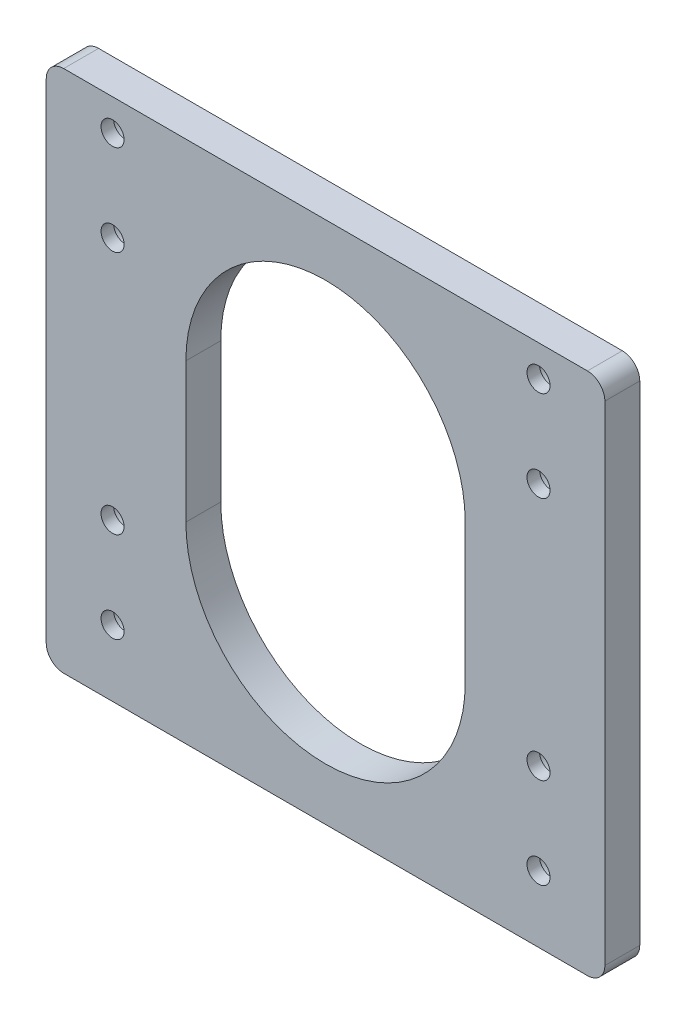
from build123d import *

# Parameters (mm, degrees)
SKETCH_1_W                   = 160
SKETCH_1_H                   = 150
EXTRUDE_1_DEPTH              = 10
FILLET_1_R                   = 5
HOLE_WIZARD_M6_1_D           = 6.6
HOLE_WIZARD_M6_1_DEPTH       = 11.5
HOLE_WIZARD_M6_1_CBORE_D     = 11
HOLE_WIZARD_M6_1_CBORE_DEPTH = 6.4
HOLE_WIZARD_M6_1_TIP         = 1.982840043
CUT_EXTRUDE_1_DEPTH          = 10


with BuildPart() as part:
    # 草图1 → 凸台-拉伸1 (new body)
    with BuildSketch(Plane.XY):
        with Locations((28963.620313483, 18.565660066)):
            Rectangle(SKETCH_1_W, SKETCH_1_H)
    extrude(amount=EXTRUDE_1_DEPTH)

    # 圆角1
    fillet_1_edges = [part.edges().sort_by_distance(p)[0] for p in [
        (28883.620313483, 93.565660066, 5),
        (29043.620313483, 93.565660066, 5),
        (29043.620313483, -56.434339934, 5),
        (28883.620313483, -56.434339934, 5),
    ]]
    fillet(fillet_1_edges, radius=FILLET_1_R)

    # M6 六角凹头螺钉的柱形沉头孔1
    with Locations(Plane(origin=(0, 0, 0), x_dir=(-1, 0, 0), z_dir=(0, 0, -1))):
        with Locations((-29024.620313483, 84.565660077), (-29024.620313483, 58.565660077), (-29024.620313483, -11.434339923), (-29024.620313483, -37.434339923), (-28902.620313482, -37.434339923), (-28902.620313482, -11.434339923), (-28902.620313482, 58.565660077), (-28902.620313482, 84.565660077)):
            CounterBoreHole(HOLE_WIZARD_M6_1_D / 2, HOLE_WIZARD_M6_1_CBORE_D / 2, HOLE_WIZARD_M6_1_CBORE_DEPTH, depth=HOLE_WIZARD_M6_1_DEPTH)
            with Locations((0, 0, -(HOLE_WIZARD_M6_1_DEPTH + HOLE_WIZARD_M6_1_TIP / 2))):  # 118° drill point
                Cone(0, HOLE_WIZARD_M6_1_D / 2, HOLE_WIZARD_M6_1_TIP, mode=Mode.SUBTRACT)

    # 草图4 → 切除-拉伸1 (cut)
    with BuildSketch(Plane.XY.offset(10)):
        with BuildLine():
            Line((28923.620313483, -1.434339933), (28923.620313483, 38.565660067))
            ThreePointArc((28923.620313483, 38.565660067), (28963.620313483, 78.565660067), (29003.620313483, 38.565660067))
            Line((29003.620313483, 38.565660067), (29003.620313483, -1.434339933))
            ThreePointArc((29003.620313483, -1.434339933), (28963.620313483, -41.434339933), (28923.620313483, -1.434339933))
        make_face()
    extrude(amount=-CUT_EXTRUDE_1_DEPTH, mode=Mode.SUBTRACT)


solid = part.part
